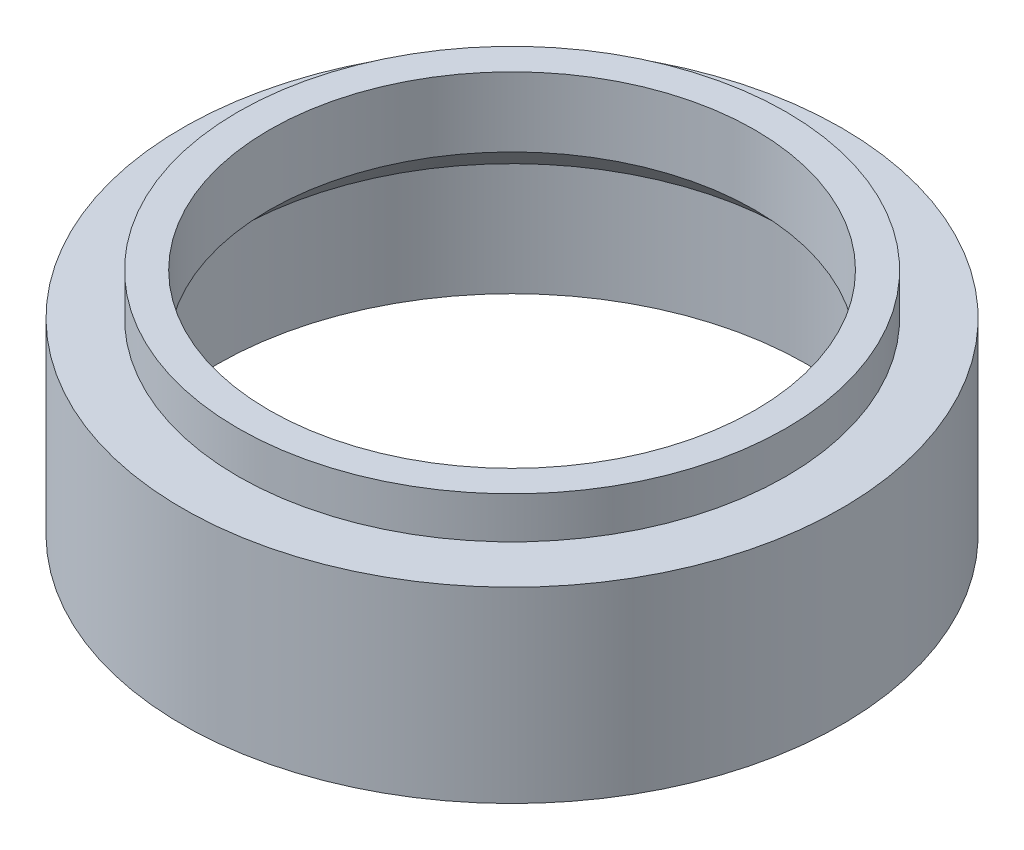
SolidWorks part; units mm, degrees
material "6061 合金"
ref_plane "前视基准面" through (0, 0, 0) normal (0, 0, 1) x (1, 0, 0)
ref_plane "上视基准面" through (0, 0, 0) normal (0, 1, 0) x (1, 0, 0)
ref_plane "右视基准面" through (0, 0, 0) normal (1, 0, 0) x (0, 0, -1)
sketch "草图2" plane through (0, 0, 0) normal (0, 0, 1) x (1, 0, 0)
  line L0 (0, 0) -> (0, 48.9157) construction
  line L1 (-35, 33) -> (-39.5, 33)
  line L2 (-39.5, 33) -> (-39.5, 27)
  line L3 (-39.5, 27) -> (-47.5, 27)
  line L4 (-47.5, 27) -> (-47.5, 0)
  line L5 (-47.5, 0) -> (-42.5, 0)
  line L6 (-42.5, 0) -> (-42.5, 18)
  line L7 (-42.5, 18) -> (-35, 18)
  line L8 (-35, 18) -> (-35, 33)
  dimension "D1" = 6
  dimension "D2" = 27
  dimension "D3" = 39.5
  dimension "D4" = 42.5
  dimension "D5" = 18
  dimension "D6" = 35
  dimension "D7" = 47.5
  dimension "D8" = 0
revolve "旋转1" add sketch "草图2" angle 360 about L0
chamfer "倒角1" distance 5 angle 45 1 edges at (0, 18, -35)
